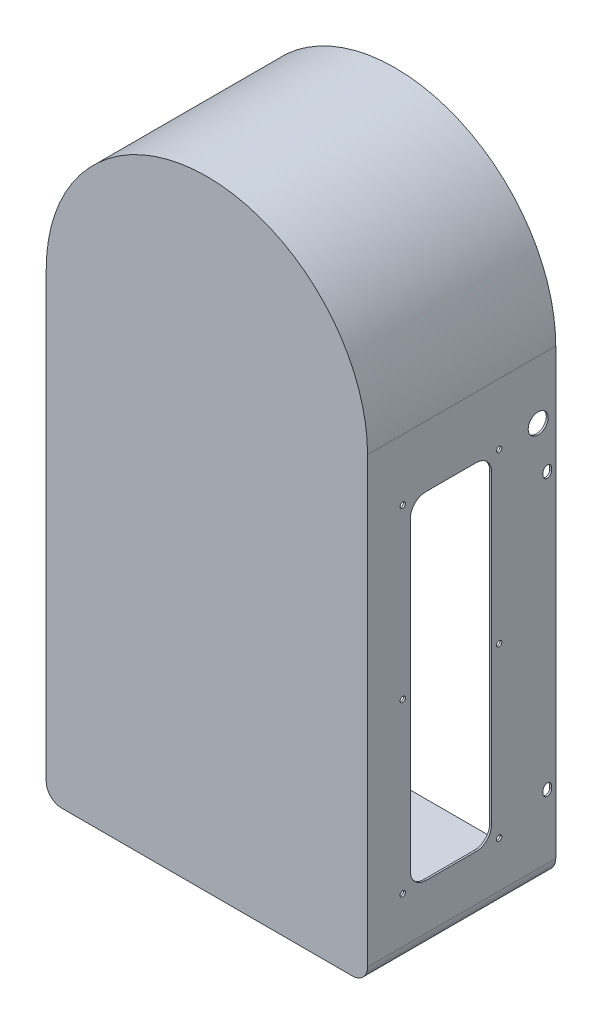
from build123d import *

# Parameters (mm, degrees)
BOSS_EXTRUDE1_DEPTH = 123
BOSS_EXTRUDE2_START = -1.2
BOSS_EXTRUDE2_DEPTH = 1.2
FILLET1_R           = 10
FILLET2_R           = 10
CUT_EXTRUDE1_DEPTH  = 353.063005725
SKETCH4_R           = 6.5
CUT_EXTRUDE2_DEPTH  = 353.063005725
SKETCH5_W           = 53
SKETCH5_H           = 220
CUT_EXTRUDE3_DEPTH  = 353.063005725
FILLET3_R           = 10
SKETCH6_R           = 1.75
CUT_EXTRUDE4_DEPTH  = 353.063005725


with BuildPart() as part:
    # Sketch1 → Boss-Extrude1 (new body)
    with BuildSketch(Plane.XY):
        with BuildLine():
            Line((-105, -150.6), (-105, 149.4))
            ThreePointArc((-105, 149.4), (0, 254.4), (105, 149.4))
            Line((105, 149.4), (105, -150.6))
            Line((105, -150.6), (-105, -150.6))
        make_face()
        with BuildLine():
            Line((93.8, -149.4), (-93.8, -149.4))
            ThreePointArc((-93.8, -149.4), (-100.871067812, -146.471067812), (-103.8, -139.4))
            Line((-103.8, -139.4), (-103.8, 149.4))
            ThreePointArc((-103.8, 149.4), (0, 253.2), (103.8, 149.4))
            Line((103.8, 149.4), (103.8, -139.4))
            ThreePointArc((103.8, -139.4), (100.871067812, -146.471067812), (93.8, -149.4))
        make_face(mode=Mode.SUBTRACT)
    extrude(amount=BOSS_EXTRUDE1_DEPTH)

    # Sketch2 → Boss-Extrude2 (add)
    with BuildSketch(Plane.XY.offset(123).offset(BOSS_EXTRUDE2_START)):
        with BuildLine():
            Line((-105, 149.4), (-105, -150.6))
            Line((-105, -150.6), (105, -150.6))
            Line((105, -150.6), (105, 149.4))
            ThreePointArc((105, 149.4), (0, 254.4), (-105, 149.4))
        make_face()
    extrude(amount=BOSS_EXTRUDE2_DEPTH)

    # Fillet1
    fillet1_edges = [part.edges().sort_by_distance(p)[0] for p in [
        (-105, -150.6, 61.5),
    ]]
    fillet(fillet1_edges, radius=FILLET1_R)

    # Fillet2
    fillet2_edges = [part.edges().sort_by_distance(p)[0] for p in [
        (105, -150.6, 61.5),
    ]]
    fillet(fillet2_edges, radius=FILLET2_R)

    # Sketch3 → Cut-Extrude1 (cut, through all)
    with BuildSketch(Plane.ZY.offset(105)):
        with BuildLine():
            Line((2.75, 80.1), (2.75, 82.1))
            ThreePointArc((2.75, 82.1), (5.5, 84.85), (8.25, 82.1))
            Line((8.25, 82.1), (8.25, 80.1))
            ThreePointArc((8.25, 80.1), (5.5, 77.35), (2.75, 80.1))
        make_face()
        with BuildLine():
            Line((2.75, -99.9), (2.75, -97.9))
            ThreePointArc((2.75, -97.9), (5.5, -95.15), (8.25, -97.9))
            Line((8.25, -97.9), (8.25, -99.9))
            ThreePointArc((8.25, -99.9), (5.5, -102.65), (2.75, -99.9))
        make_face()
    extrude(amount=-CUT_EXTRUDE1_DEPTH, mode=Mode.SUBTRACT)

    # Sketch4 → Cut-Extrude2 (cut, through all)
    with BuildSketch(Plane.ZY.offset(105)):
        with Locations(Location((11.5, 111.4, 0), (0, 0, 270))):
            Circle(SKETCH4_R)
    extrude(amount=-CUT_EXTRUDE2_DEPTH, mode=Mode.SUBTRACT)

    # Sketch5 → Cut-Extrude3 (cut, through all)
    with BuildSketch(Plane(origin=(105, 0, 0), x_dir=(0, 0, -1), z_dir=(1, 0, 0))):
        with Locations((-68.5, -0.6)):
            Rectangle(SKETCH5_W, SKETCH5_H)
    extrude(amount=-CUT_EXTRUDE3_DEPTH, mode=Mode.SUBTRACT)

    # Fillet3
    fillet3_edges = [part.edges().sort_by_distance(p)[0] for p in [
        (-104.4, 109.4, 95),
        (-104.4, 109.4, 42),
        (-104.4, -110.6, 42),
        (-104.4, -110.6, 95),
        (104.4, 109.4, 95),
        (104.4, 109.4, 42),
        (104.4, -110.6, 42),
        (104.4, -110.6, 95),
    ]]
    fillet(fillet3_edges, radius=FILLET3_R)

    # Sketch6 → Cut-Extrude4 (cut, through all)
    with BuildSketch(Plane(origin=(105, 0, 0), x_dir=(0, 0, -1), z_dir=(1, 0, 0))):
        with Locations(Location((-37, 109.4, 0), (0, 0, 90))):
            Circle(SKETCH6_R)
        with Locations(Location((-37, -0.6, 0), (0, 0, 90))):
            Circle(SKETCH6_R)
        with Locations(Location((-37, -110.6, 0), (0, 0, 90))):
            Circle(SKETCH6_R)
        with Locations(Location((-100, -110.6, 0), (0, 0, 90))):
            Circle(SKETCH6_R)
        with Locations(Location((-100, -0.6, 0), (0, 0, 90))):
            Circle(SKETCH6_R)
        with Locations(Location((-100, 109.4, 0), (0, 0, 90))):
            Circle(SKETCH6_R)
    extrude(amount=-CUT_EXTRUDE4_DEPTH, mode=Mode.SUBTRACT)


solid = part.part
